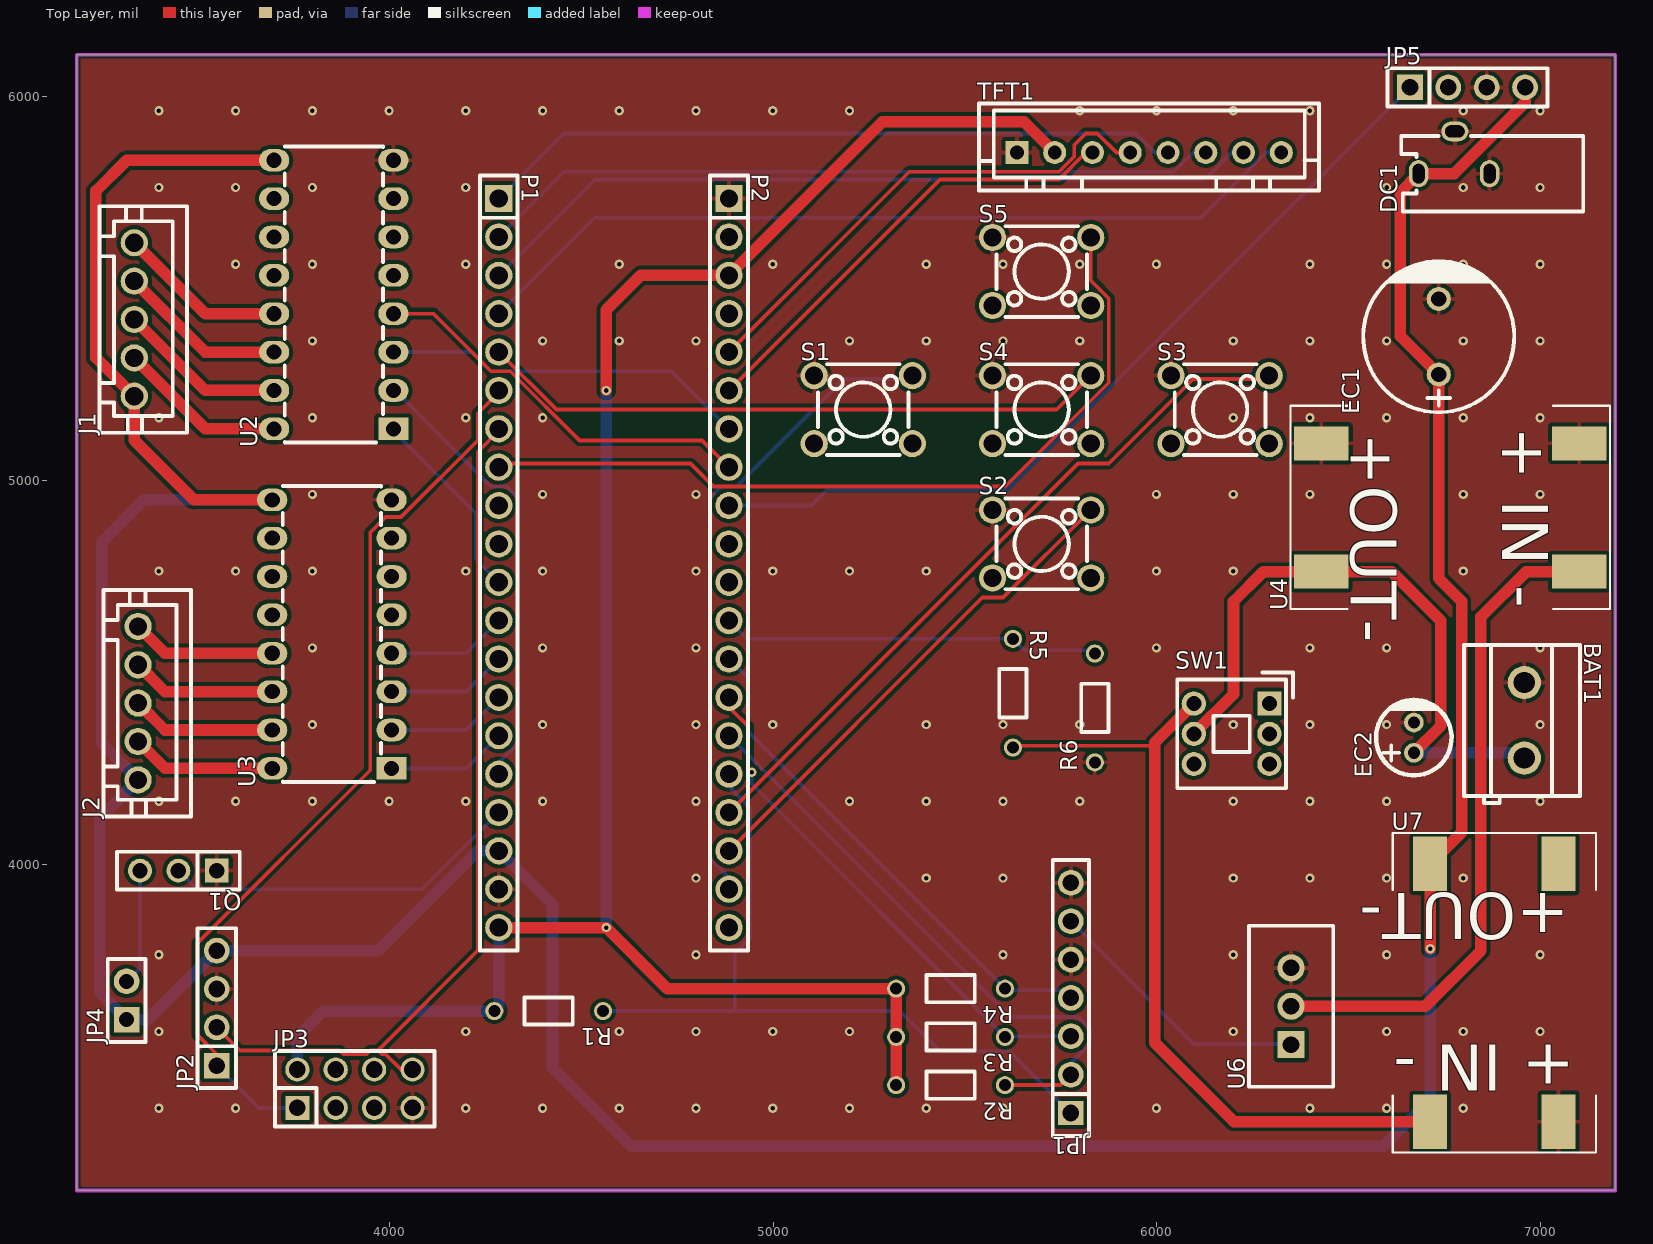
[diagram p0: Top Layer view]
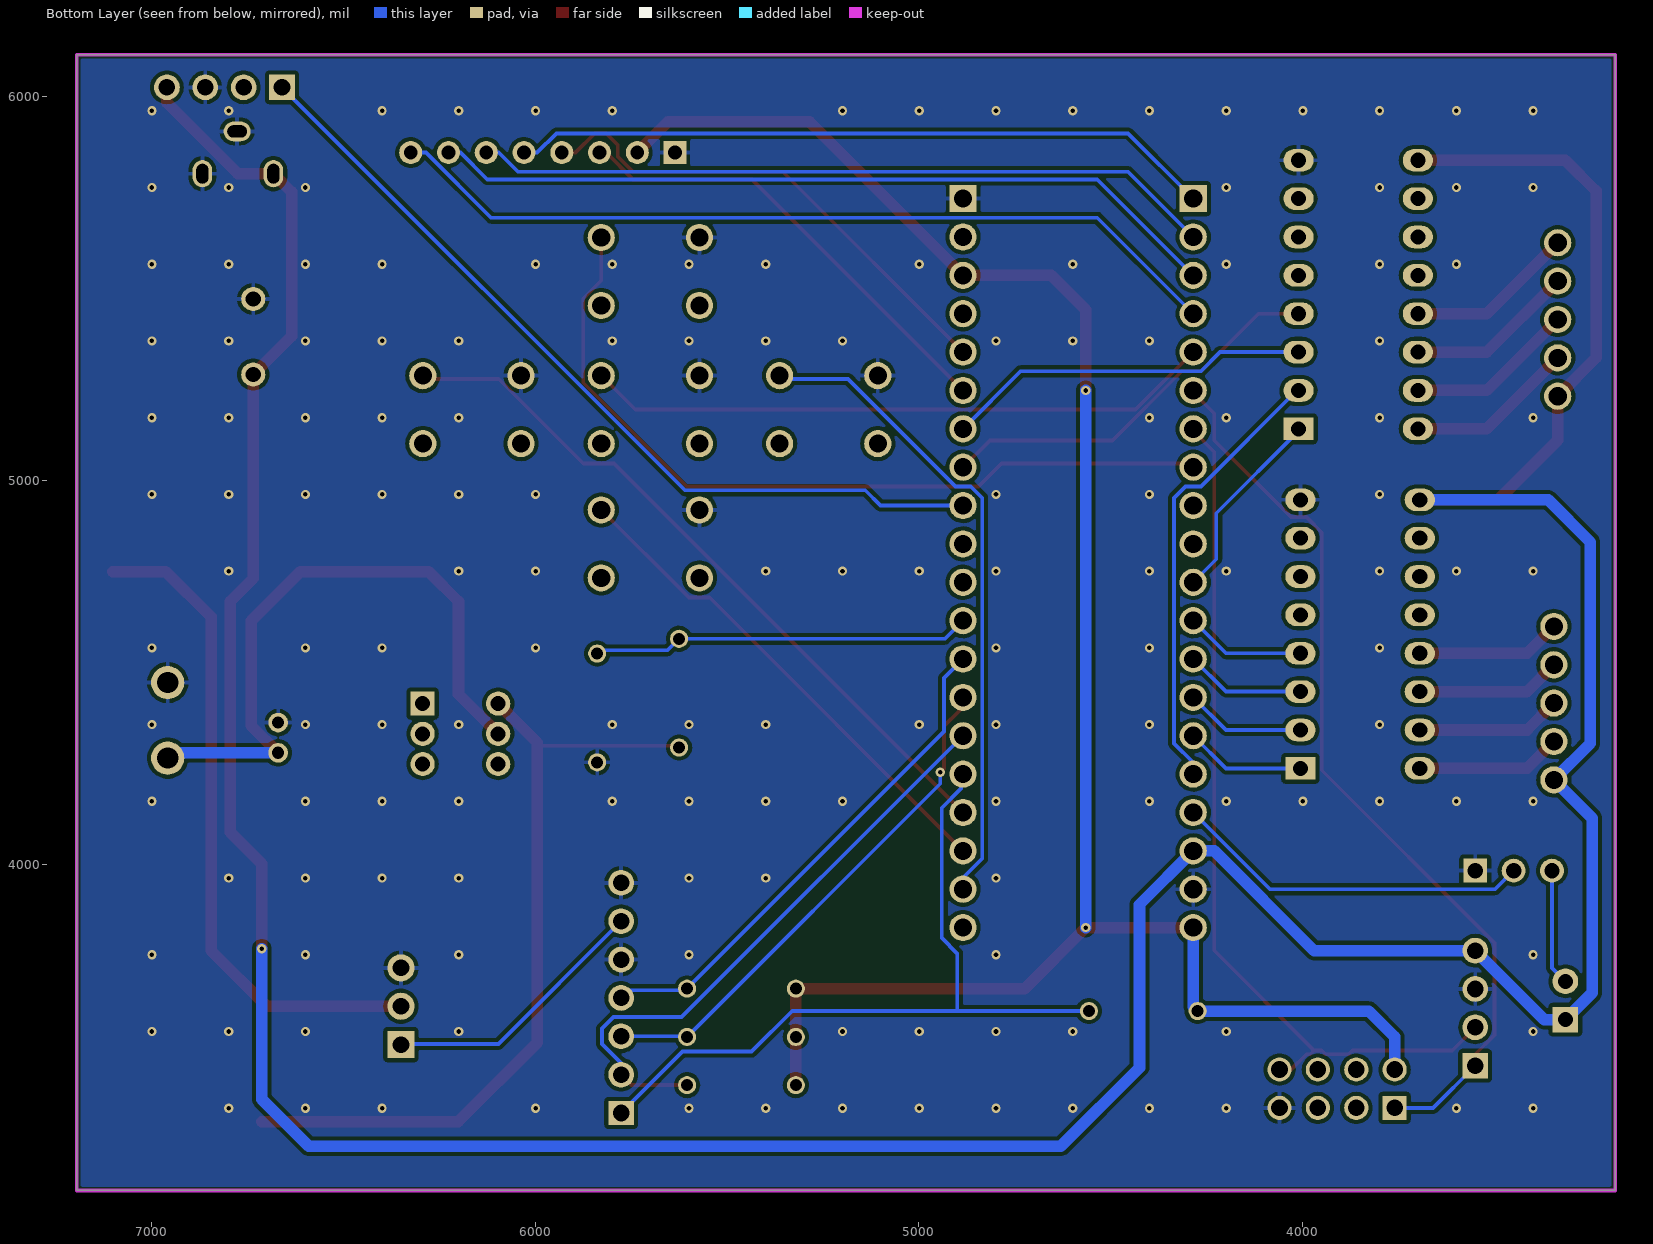
[diagram p1: Bottom Layer view, seen from below]
# Altium PCB MISC51567.pcbdoc
Units mil, origin at the board's own origin, x right, y up, seen from the top; angles counter-clockwise.
Board outline 4010 x 2960 mil, 2 copper layers (Top Layer, Bottom Layer), stack 62.206 mil thick; 32 components, 47 nets, 176 pads, 153 vias.

## Layer stack, top to bottom
Top Solder Mask Layer: solder mask 0.394, Dk 3.3
Top Layer: signal copper 1.379
Dielectric1: surface 59.449, FR4, Dk 4.5
Bottom Layer: signal copper 1.378
Bottom Solder Mask Layer: solder mask 0.394, Dk 3.3

## Board outline
3185,6110 3185,3150 7195,3150 7195,6110

## Design rules (kind name [scope] priority, off if disabled: settings)
BoardOutlineClearance copperThickness2oz_1 [All] p2 off: genericclearance=7.99 ignorepadtopadclearanceinfootprint=FALSE except(0: Arc-SplitContinuation Track-SplitContinuation SMDPad-SplitContinuation THPad-SplitContinuation Via-SplitContinuation Fill-SplitContinuation Region-SplitContinuation Poly-SplitContinuation Text-SplitContinuation Hole-SplitContinuation; 5.98: Arc-CutoutEdge SMDPad-CutoutEdge THPad-CutoutEdge Via-CutoutEdge Fill-CutoutEdge Region-CutoutEdge Text-CutoutEdge; 6.93: Hole-OutlineEdge Hole-CutoutEdge; 10: Poly-OutlineEdge Poly-CutoutEdge; 11.81: Arc-OutlineEdge Track-OutlineEdge SMDPad-OutlineEdge THPad-OutlineEdge Via-OutlineEdge Fill-OutlineEdge Region-OutlineEdge Text-OutlineEdge Track-CutoutEdge)
BoardOutlineClearance copperThickness1oz_1 [All] p4: genericclearance=4.02 ignorepadtopadclearanceinfootprint=FALSE except(0: Arc-SplitContinuation Track-SplitContinuation SMDPad-SplitContinuation THPad-SplitContinuation Via-SplitContinuation Fill-SplitContinuation Region-SplitContinuation Poly-SplitContinuation Text-SplitContinuation Hole-SplitContinuation; 6: SMDPad-CutoutEdge THPad-CutoutEdge Via-CutoutEdge Fill-CutoutEdge Region-CutoutEdge Text-CutoutEdge; 6.93: Hole-OutlineEdge Hole-CutoutEdge; 10: Poly-OutlineEdge Poly-CutoutEdge; 11.8: Arc-OutlineEdge Track-OutlineEdge SMDPad-OutlineEdge THPad-OutlineEdge Via-OutlineEdge Fill-OutlineEdge Region-OutlineEdge Text-OutlineEdge; 11.81: Arc-CutoutEdge Track-CutoutEdge)
Clearance copperThickness2oz [All] p1 off: gap=7.99 ignorepadtopadclearanceinfootprint=FALSE except(5.98: SMDPad-Track SMDPad-SMDPad THPad-Track SMDPad-THPad THPad-THPad Track-Via SMDPad-Via THPad-Via Via-Via Fill-Track Region-Track Fill-SMDPad Region-SMDPad Fill-THPad Region-THPad Fill-Via Region-Via Fill-Fill Fill-Region Region-Region Arc-Track Arc-SMDPad Arc-THPad Arc-Via Fill-Arc Region-Arc Arc-Arc Text-Track SMDPad-Text Text-THPad Text-Via Fill-Text Region-Text Arc-Text Text-Text; 6.93: Hole-Track Hole-SMDPad Hole-THPad Hole-Via Fill-Hole Region-Hole Hole-Arc Hole-Text; 10: Poly-Track Poly-SMDPad Poly-THPad Poly-Via Poly-Fill Poly-Region Poly-Poly Poly-Arc Poly-Text Poly-Hole)
Clearance copperThickness1oz [All] p3: gap=4.02 ignorepadtopadclearanceinfootprint=FALSE except(5.98: SMDPad-Track SMDPad-SMDPad THPad-Track SMDPad-THPad THPad-THPad Track-Via SMDPad-Via THPad-Via Via-Via Fill-Track Region-Track Fill-SMDPad Region-SMDPad Fill-THPad Region-THPad Fill-Via Region-Via Fill-Fill Fill-Region Region-Region; 6: Arc-Track Arc-SMDPad Arc-THPad Arc-Via Fill-Arc Region-Arc Arc-Arc Text-Track SMDPad-Text Text-THPad Text-Via Fill-Text Region-Text Arc-Text Text-Text; 6.93: Hole-Track Hole-SMDPad Hole-THPad Hole-Via Fill-Hole Region-Hole Hole-Arc Hole-Text; 10: Poly-Track Poly-SMDPad Poly-THPad Poly-Via Poly-Fill Poly-Region Poly-Poly Poly-Arc Poly-Text Poly-Hole)
DiffPairsRouting differentialPair [All] p1: maxlimit=6 minlimit=6 mostfreqgap=6 toplayer_minwidth=5 toplayer_prefwidth=10 toplayer_maxwidth=100 toplayer_mingap=6 toplayer_prefgap=6 toplayer_maxgap=6 bottomlayer_minwidth=5 bottomlayer_prefwidth=10 bottomlayer_maxwidth=100 bottomlayer_mingap=6 bottomlayer_prefgap=6 bottomlayer_maxgap=6 maxuncoupledlength=10
HoleToHoleClearance otherClearance [All] p1: gap=11.81 allowstackedmicrovias=TRUE
Length netLength [All] p1: minlimit=0 maxlimit=0
MatchedLengths netLengthTolerance [All] p1: tolerance=1000
PasteMaskExpansion pasteMaskExpansion [All] p1: expansion=0
PlaneConnect innerPlane [All] p1: planeconnectstyle=Relief reliefexpansion=20 reliefentries=4 reliefconductorwidth=10 reliefairgap=10
PolygonConnect copperRegion [(InNet('GND'))] p1: connectstyle=Relief reliefconductorwidth=10 reliefentries=4 polygonreliefangle="90 Angle" airgapwidth=10 via.connectstyle=Relief via.reliefconductorwidth=10 via.reliefentries=4 via.polygonreliefangle="90 Angle" via.airgapwidth=10
RoutingVias viaSize [All] p1: holewidth=12.01 width=24.02 viastyle="Through Hole" minholewidth=11.81 minwidth=19.68 maxholewidth=248.03 maxwidth=393.7
SolderMaskExpansion solderMaskExpansion [IsVia] p1: expansion=-1000 istentingtop=TRUE
SolderMaskExpansion solderMaskExpansion [All] p2: expansion=2 istentingtop=FALSE
Width copperThickness2oz_2 [All] p1 off: maxlimit=100 minlimit=8 preferedwidth=10
Width copperThickness1oz_2 [All] p2: maxlimit=100 minlimit=5 preferedwidth=10

## Components (designator, comment, footprint, x,y, rotation, side; value= is the part's Value field where it differs from the comment)
BAT1 "Li-battery interface" CONN-TH_2P-P5.00_KF301-2P 6957.89,4375.02 r270 top
DC1 "DC002-1.3" DC-IN-TH_DC002-1.3 6775,5855 r90 top
EC1 "220uF" CAP-TH_BD10.0-P5.00-D0.6-FD 6735,5375 r90 top
EC2 "10uF" CAP-TH_BD5.0-P2.00-D0.8-FD-10UF50VC110GL 6670,4330 r90 top
J1 "Stepper motor" CONN-TH_5P-P2.54_C9900008095 3335,5420 r90 top
J2 "Stepper motor" CONN-TH_5P-P2.54_C9900008095 3345,4420 r90 top
JP1 "HDR-1X7" HDR-TH_7P-P2.54-V-F 5776.1,3651.65 r90 top
JP2 "HDR-1X4" HDR-TH_4P-P2.54-V-F 3550,3625 r90 top
JP3 "Header 4X2" HDR-TH_8P-P2.54-V-F-R2-C4-S2.54-1 3910,3415 r0 top
JP4 "HDR-1X2" HDR-TH_2P-P2.54-V-F 3315,3645 r90 top
JP5 "HDR-1X4" HDR-TH_4P-P2.54-V-F 6810,6025 r0 top
P1 "Header 20" HDR-TH_20P-P2.54-V-F 4285,4785 r270 top
P2 "header20-1" HDR-TH_20P-P2.54-V-F 4885,4785 r270 top
Q1 "SS8050" HDR-TH_3P-P2.54-V-F 3449.89,3983.56 r180 top
R1 "10K" Res_1/8W 4415,3620 r180 top
R2 "10K" Res_1/8W 5462.5,3426.8 r180 top
R3 "10K" Res_1/8W 5462.5,3552.55 r180 top
R4 "10K" Res_1/8W 5462.5,3678.29 r180 top
R5 "10K" Res_1/8W 5622.48,4446.01 r270 top
R6 "10K" Res_1/8W 5841.01,4407.47 r90 top
S1 "BUTTOM" SW-TH_4P-L6.0-W6.0-P4.50-LS6.5 5235,5185 r0 top
S2 "BUTTOM" SW-TH_4P-L6.0-W6.0-P4.50-LS6.5 5700,4835 r0 top
S3 "BUTTOM" SW-TH_4P-L6.0-W6.0-P4.50-LS6.5 6165,5185 r0 top
S4 "BUTTOM" SW-TH_4P-L6.0-W6.0-P4.50-LS6.5 5700,5185 r0 top
S5 "BUTTOM" SW-TH_4P-L6.0-W6.0-P4.50-LS6.5 5700,5545 r0 top
SW1 "Self-lock button" SW-TH_6P-L7.0-W7.0-P2.00 6195,4340 r0 top
TFT1 "TFT-1.44" CONN-TH_8P-P2.50_ZX-XH2.54-8PZZ-GW 5980,5855 r0 top
U2 "ULN2003" PDIP-16_L19.6-W6.5-P2.54-LS7.9-BL 3855,5485 r90 top
U3 "ULN2003" PDIP-16_L19.6-W6.5-P2.54-LS7.9-BL 3850,4600 r90 top
U4 "Li-battery charge MODE" JYMK 6765,4930 r90 top
U6 "AMS117-05" CONN-TH_3P-P2.54_8-102202-4 6350,3630 r90 top
U7 "Li-battery boost MODE" JYMK 6880,3665 r0 top

## Footprints (in the part's own frame and the unit in brackets; to place one, negate y for a bottom-side part, rotate by r counter-clockwise, add the part's x,y. Pads: shape width x height; smd on the part's side, far side on the other; paste and mask are expansions set on the pad)
CAP-TH_BD5.0-P2.00-D0.8-FD-10UF50VC110GL [mm]
  round 1.3 hole 0.8: 1(-1,0) 2(1,0)
  silkscreen extent -2.5,-2.5 2.5,2.5
CAP-TH_BD10.0-P5.00-D0.6-FD [mm]
  round 1.6 hole 1 paste+0 mask+0.05: 1(-2.5,0) 2(2.5,0)
  silkscreen extent -5,-5 5.08,5
CONN-TH_2P-P5.00_KF301-2P [mm]
  round 2.2 hole 1.4: 1(-2.5,0) 2(2.5,0)
  silkscreen extent -5,-4 5.46,3.7
CONN-TH_3P-P2.54_8-102202-4 [mm]
  rect 1.8x1.8 hole 1.1: 1(-2.54,0)
  round 1.8 hole 1.1: 2(0,0) 3(2.54,0)
  silkscreen extent -5.33,-2.79 5.33,2.79
CONN-TH_5P-P2.54_C9900008095 [mm]
  round 1.8 hole 1.2 paste+0 mask+0.05: 1(-5.08,0) 2(-2.54,0) 3(0,0) 5(5.08,0)
  round 1.8 hole 1.2 copper offset 0,0 paste+0 mask+0.05: 4(2.54,0)
  silkscreen extent -7.5,-3.5 7.5,2.3
CONN-TH_8P-P2.50_ZX-XH2.54-8PZZ-GW [mil]
  rect 60x60 hole 36: 1(-344.49,0)
  round 60 hole 36: 2(-246.06,0) 3(-147.64,0) 4(-49.22,0) 5(49.21,0) 6(147.64,0) 7(246.06,0) 8(344.48,0)
  silkscreen extent -443,-98 443,128
DC-IN-TH_DC002-1.3 [mm]
  oval 1.8x1.3 hole 0.8 slot 1.3 at 0 deg paste+0 mask+0.05: 1(-1.4,2.35) 3(-1.4,-2.35)
  oval 1.3x1.8 hole 0.8 slot 1.3 at 90 deg paste+0 mask+0.05: 2(1.4,-0.05)
  silkscreen extent -3.9,-8.55 1.1,3.5
HDR-TH_2P-P2.54-V-F [mm]
  rect 1.7x1.7 hole 1: 1(-1.27,0)
  round 1.7 hole 1: 2(1.27,0)
  silkscreen extent -2.74,-1.25 2.74,1.25
HDR-TH_3P-P2.54-V-F [mil]
  rect 62x62 hole 40.16: 1(-100,0)
  round 62 hole 40.16: 2(0,0) 3(100,0)
  silkscreen extent -160,-49 160,49
HDR-TH_4P-P2.54-V-F [mm]
  rect 1.7x1.7 hole 1.1: 1(-3.81,0)
  round 1.7 hole 1.1: 2(-1.27,0) 3(1.27,0) 4(3.81,0)
  silkscreen extent -5.29,-1.27 5.29,1.27
HDR-TH_7P-P2.54-V-F [mm]
  rect 1.575x1.7 hole 1.1: 1(-7.62,0)
  round 1.7 hole 1.1: 2(-5.08,0) 3(-2.54,0) 4(0,0) 5(2.54,0) 6(5.08,0) 7(7.62,0)
  silkscreen extent -9.13,-1.2 9.13,1.2
HDR-TH_8P-P2.54-V-F-R2-C4-S2.54-1 [mm]
  rect 1.6x1.6 hole 1.1: 1(-3.81,-1.27)
  round 1.6 hole 1.1: 2(-3.81,1.27) 3(-1.27,-1.27) 4(-1.27,1.27) 5(1.27,-1.27) 6(1.27,1.27) 7(3.81,-1.27) 8(3.81,1.27)
  silkscreen extent -5.28,-2.5 5.28,2.5
HDR-TH_20P-P2.54-V-F [mm]
  rect 1.8x1.8 hole 1.2: 1(-24.13,0)
  round 1.8 hole 1.2: 2(-21.59,0) 3(-19.05,0) 4(-16.51,0) 5(-13.97,0) 6(-11.43,0) 7(-8.89,0) 8(-6.35,0) 9(-3.81,0) 10(-1.27,0) 11(1.27,0) 12(3.81,0) 13(6.35,0) 14(8.89,0) 15(11.43,0) 16(13.97,0) 17(16.51,0) 18(19.05,0) 19(21.59,0) 20(24.13,0)
  silkscreen extent -25.65,-1.25 25.65,1.25
JYMK [mm]
  rect 2.25x3.625 smd: 1(-4.25,-8.537) 2(4.25,-8.537) 3(4.25,8.537) 4(-4.25,8.537)
  silkscreen extent -6.73,-10.58 6.73,10.58
PDIP-16_L19.6-W6.5-P2.54-LS7.9-BL [mm]
  rect 1.5x2 hole 1: 1(-8.89,-3.95)
  oval 1.5x2 hole 1: 2(-6.35,-3.95) 3(-3.81,-3.95) 4(-1.27,-3.95) 5(1.27,-3.95) 6(3.81,-3.95) 7(6.35,-3.95) 8(8.89,-3.95) 9(8.89,3.95) 10(6.35,3.95) 11(3.81,3.95) 12(1.27,3.95) 13(-1.27,3.95) 14(-3.81,3.95) 15(-6.35,3.95) 16(-8.89,3.95)
  silkscreen extent -9.8,-3.25 9.8,3.25
Res_1/8W [mil]
  round 47.2 hole 31.5 paste+0 mask+2: 1(-141.7,2.48) 2(141.7,2.48)
  silkscreen extent -63,-33 63,38
SW-TH_4P-L6.0-W6.0-P4.50-LS6.5 [mm]
  round 1.8 hole 1.2: 1(-3.25,2.25) 2(3.25,2.25) 3(-3.25,-2.25) 4(3.25,-2.25)
  silkscreen extent -3,-3 3,3
SW-TH_6P-L7.0-W7.0-P2.00 [mm]
  rect 1.6x1.6 hole 1: 1(2.5,2)
  round 1.6 hole 1: 2(2.5,0) 3(2.5,-2) 4(-2.5,2) 5(-2.5,0) 6(-2.5,-2)
  silkscreen extent -3.6,-3.6 4.06,4.06

## Via types
v1: diameter 24.02, hole 12, Top Layer to Bottom Layer, 153 vias

## Nets (pads, with @x,y where several pads share a name; then routed paths per layer and width w, separated by ;. In a path a pad name is that pad's centre, name@x,y a point inside that pad or via, vN(x,y) a via of type N, cw(c..) or ccw(c..) an arc to the next point about the centre after c; other vN are vias at no path point)
$2N72: J1.2 U2.16 | length 441.1
  Top Layer w30: J1.2 3520,5135 U2.16
$2N73: J1.3 U2.15 | length 441.1
  Top Layer w30: J1.3 3520,5235 U2.15
$2N74: J1.4 U2.14 | length 441.1
  Top Layer w30: J1.4 3520.01,5335 U2.14
$2N75: J1.5 U2.13 | length 441.1
  Top Layer w30: J1.5 3520,5435 U2.13
$2N76: J2.2 U3.16 | length 378.5
  Top Layer w30: J2.2 3415,4250 U3.16
$2N77: J2.3 U3.15 | length 378.5
  Top Layer w30: J2.3 3415,4350 U3.15
$2N78: J2.4 U3.14 | length 378.5
  Top Layer w30: J2.4 3415.01,4450 U3.14
$2N79: J2.5 U3.13 | length 378.5
  Top Layer w30: J2.5 3415,4550 U3.13
$2N80: U4.1 U6.2 | length 1729.9
  Top Layer w30: U6.2 6700,3630 6845,3775 6845,4645 6962.68,4762.68 U4.1
$2N81: BAT1.2 EC2.1 SW1.5 U4.4 | length 1680
  Top Layer w30: SW1.5 6200,4443.43 6200,4685 6277.68,4762.68 U4.4 6612.32,4762.68 6740,4635 6740,4360.63 EC2.1
  Bottom Layer w30: EC2.1 6943.86,4290.63 BAT1.2
$2N94: R5.2 SW1.4 U7.1 | length 2100.8
  Top Layer w10: R5.2 5628.11,4304.31 5632.68,4308.88 5995,4308.88
  Top Layer w30: SW1.4 5995,4317.16 5995,4308.88 5995,3535 6201.12,3328.88 U7.1
$2N106: JP5.2
$2N110: JP4.2 Q1.3 | length 303
  Bottom Layer w10: JP4.2 3349.89,3729.89 Q1.3
GND: BAT1.1 DC1.2 DC1.3 EC1.2 EC2.2 JP1.5 JP1.7 JP2.3 JP3.7 JP5.3 P1.19 P2.1 Q1.1 R6.1 S1.1 S2.1 S3.1 S4.1 S5.1 TFT1.1 U2.8 U3.8 U4.2 U4.3 U6.3 U7.2
  other v1: 3399.1,3364.1 3599.1,3364.1 4199.1,3364.1 4399.1,3364.1 4599.1,3364.1 4799.1,3364.1 4999.1,3364.1 5199.1,3364.1 5399.1,3364.1 5599.1,3364.1 5999.1,3364.1 6399.1,3364.1 6599.1,3364.1 6799.1,3364.1 3399.1,3564.1 4199.1,3564.1 4599.1,3564.1 4799.1,3564.1 4999.1,3564.1 5199.1,3564.1 6199.1,3564.1 6599.1,3564.1 6799.1,3564.1 6999.1,3564.1 3399.1,3764.1 4799.1,3764.1 5599.1,3764.1 6199.1,3764.1 6599.1,3764.1 6999.1,3764.1 4799.1,3964.1 5399.1,3964.1 5599.1,3964.1 6199.1,3964.1 6399.1,3964.1 6599.1,3964.1 6799.1,3964.1 3399.1,4164.1 3599.1,4164.1 3799.1,4164.1 3999.1,4164.1 4199.1,4164.1 4399.1,4164.1 4799.1,4164.1 5199.1,4164.1 5399.1,4164.1 5599.1,4164.1 5799.1,4164.1 6199.1,4164.1 6399.1,4164.1 6599.1,4164.1 6999.1,4164.1 3799.1,4364.1 4399.1,4364.1 4799.1,4364.1 4999.1,4364.1 5399.1,4364.1 5599.1,4364.1 5799.1,4364.1 6199.1,4364.1 6399.1,4364.1 6599.1,4364.1 6999.1,4364.1 3799.1,4564.1 4399.1,4564.1 4799.1,4564.1 5999.1,4564.1 6399.1,4564.1 6599.1,4564.1 6999.1,4564.1 3399.1,4764.1 3599.1,4764.1 3799.1,4764.1 4199.1,4764.1 4399.1,4764.1 4799.1,4764.1 4999.1,4764.1 5199.1,4764.1 5399.1,4764.1 5999.1,4764.1 6199.1,4764.1 6799.1,4764.1 3799.1,4964.1 4399.1,4964.1 4799.1,4964.1 5999.1,4964.1 6199.1,4964.1 6399.1,4964.1 6599.1,4964.1 6799.1,4964.1 6999.1,4964.1 3399.1,5164.1 3799.1,5164.1 4199.1,5164.1 4399.1,5164.1 6199.1,5164.1 6399.1,5164.1 6599.1,5164.1 6799.1,5164.1 6999.1,5164.1 3799.1,5364.1 4399.1,5364.1 4599.1,5364.1 4799.1,5364.1 5199.1,5364.1 5399.1,5364.1 5599.1,5364.1 5799.1,5364.1 6199.1,5364.1 6399.1,5364.1 6599.1,5364.1 6799.1,5364.1 6999.1,5364.1 3599.1,5564.1 3799.1,5564.1 4199.1,5564.1 4599.1,5564.1 4999.1,5564.1 5399.1,5564.1 5599.1,5564.1 5799.1,5564.1 5999.1,5564.1 6399.1,5564.1 6599.1,5564.1 6799.1,5564.1 6999.1,5564.1 3399.1,5764.1 3599.1,5764.1 3799.1,5764.1 4199.1,5764.1 6599.1,5764.1 6799.1,5764.1 6999.1,5764.1 3399.1,5964.1 3599.1,5964.1 3799.1,5964.1 3999.1,5964.1 4199.1,5964.1 4399.1,5964.1 4599.1,5964.1 4799.1,5964.1 4999.1,5964.1 5199.1,5964.1 5799.1,5964.1 5999.1,5964.1 6199.1,5964.1 6399.1,5964.1 6799.1,5964.1 6999.1,5964.1
PA0: JP1.1 P2.16 R1.1 | length 1985.9
  Bottom Layer w10: R1.1 4900.22,3617.53 ; P2.16 4890.22,4227.52 4890.22,4197.52 4940.22,4147.52 4940.22,3807.53 4900.22,3767.53 4900.22,3617.53 ; JP1.1 5616.1,3511.65 5436.1,3511.65 5330.22,3617.53 4900.22,3617.53
PA1: JP1.2 P2.15 R2.1 | length 1581.2
  Top Layer w10: R2.1 5748.77,3424.32 JP1.2
  Bottom Layer w10: P2.15 5618.35,3601.65 5796.1,3601.65 5826.1,3571.65 5826.1,3531.65 5776.1,3481.65 JP1.2
PA2: JP1.3 P2.14 R3.1 | length 1355.2
  Top Layer w10: P2.14 4884.2,4430.07 4894.2,4420.07 4894.2,4400.07 4934.2,4360.07 4934.2,4250.07 v1(4944.2,4240.07)
  Bottom Layer w10: v1(4944.2,4240.07) 4944.2,4210.07 R3.1 5616.1,3551.65 JP1.3
PA3: JP1.4 P2.13 R4.1 | length 1339
  Bottom Layer w10: P2.13 4934.2,4485.88 4934.2,4345.82 R4.1 5608.37,3671.65 5756.1,3671.65 JP1.4
PA4: P2.12 R5.1 R6.2 | length 989.1
  Bottom Layer w10: P2.12 4932.29,4587.71 R5.1 5654.96,4557.71 5830,4557.71 R6.2
PA5: P2.11
PA6: P2.10
PA7: JP5.1 P2.9 | length 2226.5
  Bottom Layer w10: P2.9 5100,4935 5140,4975 5610,4975 JP5.1
PA8: P1.5 S4.2 | length 1641.8
  Top Layer w10: P1.5 4435,5185 5739.37,5185 S4.2@5827.95,5273.58
PA9: JP2.1 JP3.1 P1.6 | length 2384.9
  Top Layer w10: JP2.1 3550,3505 3500,3555 3500,3795 3950,4245 3950,4865 3990,4905 4030,4905 4230,5105 4230,5175 4285,5230 P1.6
  Bottom Layer w10: JP2.1 3660,3365 JP3.1
PA10: JP2.2 JP3.8 P1.7 | length 2314.3
  Top Layer w10: JP2.2 3610,3515 3870,3515 3880,3505 3940,3505 3950,3515 3970,3515 ; JP3.8 4030,3465 3990,3505 3980,3505 3970,3515 ; P1.7 4285,5130 4230,5075 4230,3775 3970,3515
PA11: P1.8 S5.2 | length 2128.9
  Top Layer w10: P1.8 4295,5045 4785,5045 4845,4985 5605,4985 5875,5255 5875,5475 5827.95,5522.05 S5.2@5827.95,5633.58
PB0: P2.8 U2.4 | length 1040.2
  Top Layer w10: U2.4 4115,5435 4265,5285 4315,5285 4495,5105 4815,5105 P2.8
PB1: P2.7 U2.3 | length 957.3
  Bottom Layer w10: U2.3 4215,5335 4265,5285 4735,5285 P2.7
PB3: P1.11 U2.1 | length 513.7
  Bottom Layer w10: U2.1 4010.51,5129.49 4225,4915 4225,4795 P1.11
PB4: P1.12 U3.4 | length 314.7
  Bottom Layer w10: U3.4 4200,4550 P1.12
PB5: P1.13 U3.3 | length 314.7
  Bottom Layer w10: U3.3 4200,4450 P1.13
PB6: P1.14 U3.2 | length 314.7
  Bottom Layer w10: U3.2 4200,4350 P1.14
PB7: P1.15 U3.1 | length 314.7
  Bottom Layer w10: U3.1 4200,4250 P1.15
PB8: P1.16 U2.2 | length 1181.2
  Bottom Layer w10: U2.2 4015,5235 4265,4985 4305,4985 4335,4955 4335,4315 4285,4265 P1.16
PB9: P1.17 Q1.2 | length 938.1
  Bottom Layer w10: Q1.2 3498.45,3935 4085,3935 P1.17
PB10: P2.6 TFT1.3 | length 1204.2
  Top Layer w10: P2.6 5435,5785 5745,5785 5815,5855 TFT1.3
PB11: P2.5 TFT1.4 | length 1320.2
  Top Layer w10: P2.5 5355,5805 5745,5805 5785,5845 5785,5875 5815,5905 5845,5905 5895,5855 TFT1.4
PB12: P1.1 TFT1.5 | length 1835.3
  Bottom Layer w10: P1.1 4455,5905 5945,5905 5995,5855 TFT1.5
PB13: P1.2 TFT1.6 | length 1933.8
  Bottom Layer w10: P1.2 4455,5805 6045,5805 6095,5855 TFT1.6
PB14: P1.3 TFT1.7 | length 2073.6
  Bottom Layer w10: P1.3 4535,5785 6125,5785 6195,5855 TFT1.7
PB15: P1.4 TFT1.8 | length 2213.5
  Bottom Layer w10: P1.4 4535,5685 6115,5685 6285,5855 TFT1.8
PC13: P2.19 S1.2 | length 1700.8
  Bottom Layer w10: P2.19 4885,3965 4835,4015 4835,4955 4865,4985 4905,4985 5185,5265 5355,5265 S1.2@5362.95,5273.58
PC14: P2.18 S2.2 | length 1311
  Top Layer w10: P2.18 5545,4695 5599.37,4695 S2.2@5827.95,4923.58
PC15: P2.17 S3.2 | length 1879.8
  Top Layer w10: P2.17 5795,5045 5875,5045 6095,5265 6285,5265 S3.2@6292.95,5273.58
PV: JP1.6 U6.1 | length 706.8
  Bottom Layer w10: JP1.6 6096.1,3531.65 6346.1,3531.65 U6.1
VCC3V3: JP3.2 P1.20 P2.3 R1.2 R2.2 R3.2 R4.2 TFT1.2 | length 5216.9
  Top Layer w30: P1.20 v1(4565,3835) 4724.18,3675.82 R4.2 R3.2 R2.2 ; v1(4565,5235) 4565,5445 4655,5535 P2.3 5285,5935 5653.94,5935 TFT1.2
  Bottom Layer w30: JP3.2 3760,3550 3827.52,3617.52 R1.2 4285,3629.22 P1.20 ; v1(4565,3835) v1(4565,5235)
VCC_5V: DC1.1 EC1.1 J1.1 J2.1 JP2.4 JP4.1 JP5.4 P1.18 U2.9 U3.9 U7.4 | length 10582.7
  Top Layer w30: U3.9 3490,4950 3335,5105 J1.1 3235,5320 3235,5755 3315,5835 U2.9 ; v1(6712.68,3780) U7.4 6795,4083.44 6795,4685 6735,4745 EC1.1 6635,5376.57 6635,5752.41 DC1.1 6774.88,5799.88 6960,5985 JP5.4
  Bottom Layer w30: U3.9 3360,4950 3250,4840 3250,4315 J2.1 3245,4120 3245,3665 JP4.1 3370,3595 JP2.4 3970,3775 4230,4035 P1.18 4425,3895 4425,3470 4630,3265 6590,3265 6712.68,3387.68 v1(6712.68,3780)
pads on no net: JP3.3 JP3.4 JP3.5 JP3.6 P1.9 P1.10 P2.2 P2.4 P2.20 S1.3 S1.4 S2.3 S2.4 S3.3 S3.4 S4.3 S4.4 S5.3 S5.4 SW1.1 SW1.2 SW1.3 SW1.6 U2.5 U2.6 U2.7 U2.10 U2.11 U2.12 U3.5 U3.6 U3.7 U3.10 U3.11 U3.12 U7.3

## Polygon pours and split planes (outlines as drawn)
GND on Top Layer (solid, remove dead copper, pour order 0): 3000,6440 3000,3000 7580,3000 7580,6440
GND on Bottom Layer (solid, remove dead copper, pour order 2): 3115,6245 3115,3040 7315,3040 7315,6245

## Keep-outs
Board Outline Layer:
  the board outline again, w10